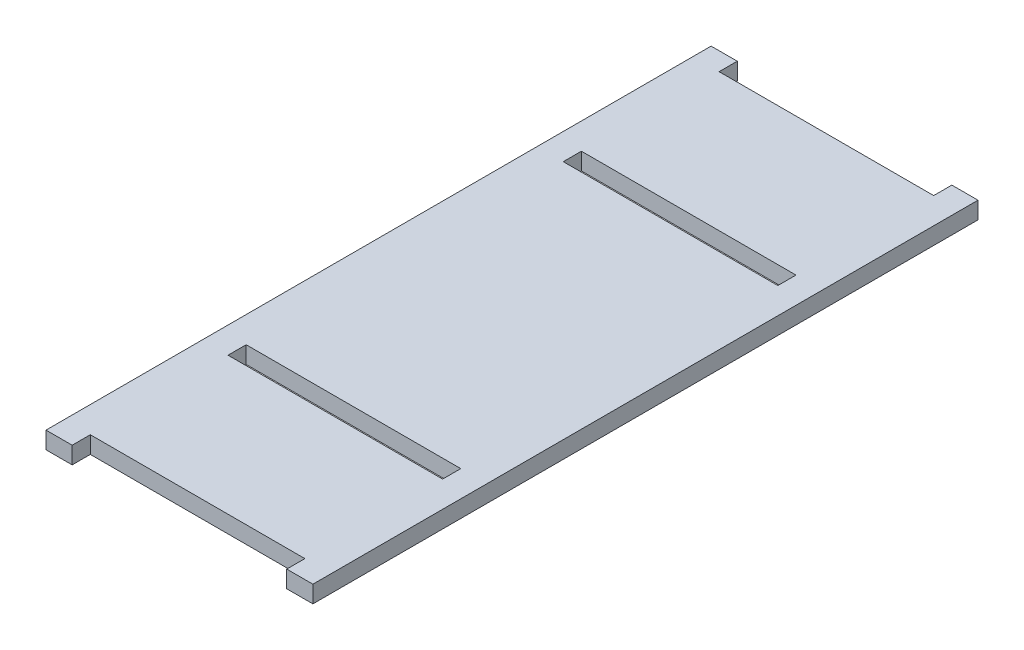
from build123d import *

# Parameters (mm, degrees)
SKETCH1_W           = 201
SKETCH1_H           = 17
BOSS_EXTRUDE1_DEPTH = 16


with BuildPart() as part:
    # Sketch1 → Boss-Extrude1 (new body)
    with BuildSketch(Plane(origin=(0, 0, 0), x_dir=(1, 0, 0), z_dir=(0, 1, 0))):
        Polygon((-125, 311.5), (-125, -311.5), (-100.5, -311.5), (-100.5, -294.5), (100.5, -294.5), (100.5, -311.5), (125, -311.5), (125, 311.5), (100.5, 311.5), (100.5, 294.5), (-100.5, 294.5), (-100.5, 311.5), align=None)
        with Locations((0, -157)):
            Rectangle(SKETCH1_W, SKETCH1_H, mode=Mode.SUBTRACT)
        with Locations((0, 157)):
            Rectangle(SKETCH1_W, SKETCH1_H, mode=Mode.SUBTRACT)
    extrude(amount=BOSS_EXTRUDE1_DEPTH)


solid = part.part
